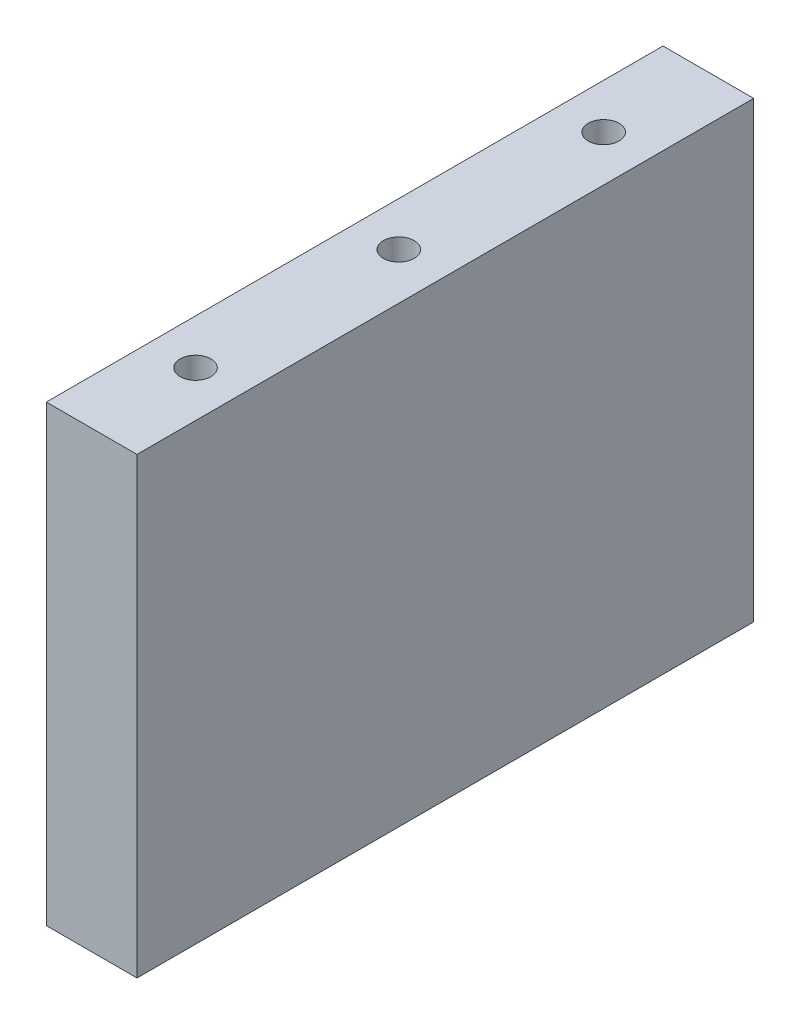
from build123d import *

# Parameters (mm, degrees)
SKETCH_1_W             = 136
SKETCH_1_H             = 100
EXTRUDE_1_DEPTH        = 20
HOLE_WIZARD_M8_1_D     = 6.8
HOLE_WIZARD_M8_1_DEPTH = 19.75
HOLE_WIZARD_M8_1_TIP   = 2.042926105
HOLE_WIZARD_M8_2_D     = 6.8
HOLE_WIZARD_M8_2_DEPTH = 19.75
HOLE_WIZARD_M8_2_TIP   = 2.042926105


with BuildPart() as part:
    # 草图1 → 凸台-拉伸1 (new body)
    with BuildSketch(Plane(origin=(0, 0, 0), x_dir=(0, 0, -1), z_dir=(1, 0, 0))):
        Rectangle(SKETCH_1_W, SKETCH_1_H)
    extrude(amount=EXTRUDE_1_DEPTH)

    # M8 螺纹孔1
    with Locations(Plane(origin=(0, 50, 0), x_dir=(1, 0, 0), z_dir=(0, 1, 0))):
        with Locations((9.910141203, 45), (9.910141203, -45), (9.734330512, 0)):
            Hole(HOLE_WIZARD_M8_1_D / 2, depth=HOLE_WIZARD_M8_1_DEPTH)
            with Locations((0, 0, -(HOLE_WIZARD_M8_1_DEPTH + HOLE_WIZARD_M8_1_TIP / 2))):  # 118° drill point
                Cone(0, HOLE_WIZARD_M8_1_D / 2, HOLE_WIZARD_M8_1_TIP, mode=Mode.SUBTRACT)

    # M8 螺纹孔2
    with Locations(Plane(origin=(0, -50, 0), x_dir=(-1, 0, 0), z_dir=(0, -1, 0))):
        with Locations((-10, 45), (-10, 0), (-10, -45)):
            Hole(HOLE_WIZARD_M8_2_D / 2, depth=HOLE_WIZARD_M8_2_DEPTH)
            with Locations((0, 0, -(HOLE_WIZARD_M8_2_DEPTH + HOLE_WIZARD_M8_2_TIP / 2))):  # 118° drill point
                Cone(0, HOLE_WIZARD_M8_2_D / 2, HOLE_WIZARD_M8_2_TIP, mode=Mode.SUBTRACT)


solid = part.part
